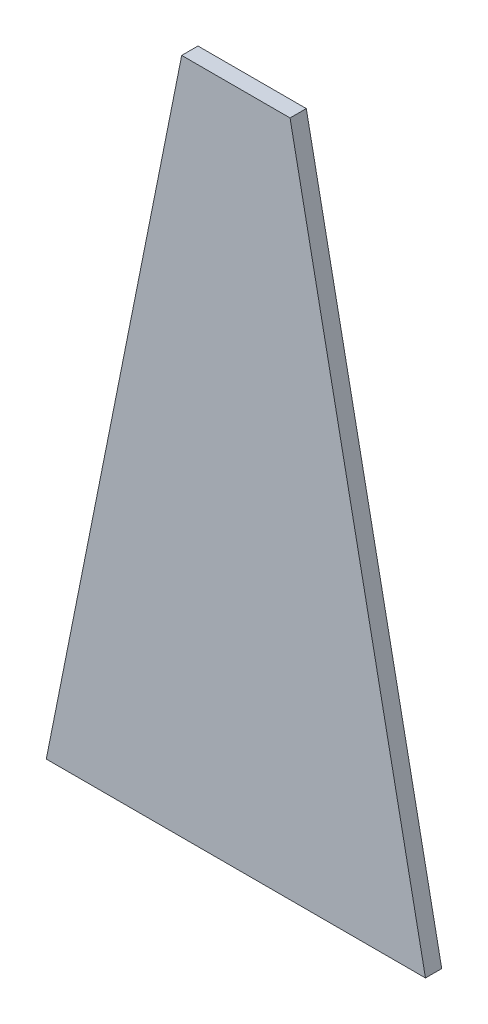
SolidWorks part; units mm, degrees
material "1023 碳钢板 (SS)"
ref_plane "前视基准面" through (0, 0, 0) normal (0, 0, 1) x (1, 0, 0)
ref_plane "上视基准面" through (0, 0, 0) normal (0, 1, 0) x (1, 0, 0)
ref_plane "右视基准面" through (0, 0, 0) normal (1, 0, 0) x (0, 0, -1)
sketch "草图1" plane through (0, 0, 0) normal (0, 0, 1) x (1, 0, 0)
  line L1 (140, 250) -> (-140, 250)
  line L2 (140, 250) -> (140, -250)
  line L3 (140, -250) -> (-140, -250)
  line L4 (-140, 250) -> (-140, -250)
  line L5 (140, 250) -> (-140, -250) construction
  line L6 (140, -250) -> (-140, 250) construction
  point P0 (0, 0)
  dimension "D1" = 280
  dimension "D2" = 500
extrude "凸台-拉伸1" add sketch "草图1" along normal blind 12
sketch "草图2" plane through (0, 0, 12) normal (0, 0, 1) x (1, 0, 0)
  line L0 (-140, -250) -> (-40, 250)
  line L1 (140, 250) -> (-140, 250) construction
  line L2 (-40, 250) -> (40, 250)
  line L3 (40, 250) -> (140, -250)
  line L4 (140, -250) -> (-140, -250)
  dimension "D1" = 80
  dimension "D2" = 100
extrude "切除-拉伸1" cut sketch "草图2" against normal blind 12 flip side to cut
